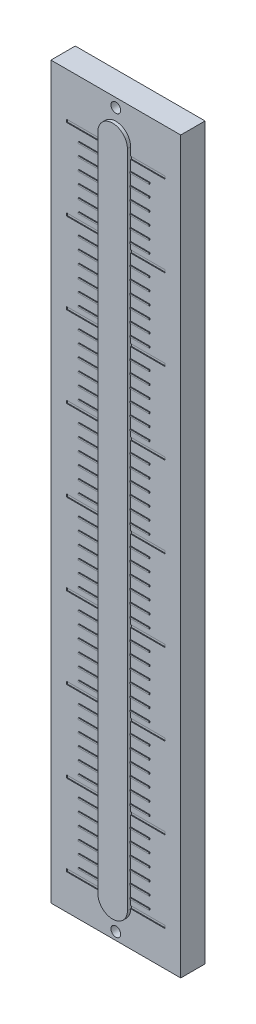
SolidWorks part; units mm, degrees
ref_plane "Front Plane" through (0, 0, 0) normal (0, 0, 1) x (1, 0, 0)
ref_plane "Top Plane" through (0, 0, 0) normal (0, 1, 0) x (1, 0, 0)
ref_plane "Right Plane" through (0, 0, 0) normal (1, 0, 0) x (0, 0, -1)
other "Configuration Table"
sketch "Sketch1" plane through (0, 0, 0) normal (0, 0, 1) x (1, 0, 0)
  line L1 (0, 0) -> (80, 0)
  line L2 (0, 0) -> (0, 450)
  line L3 (0, 450) -> (80, 450)
  line L4 (80, 0) -> (80, 450)
  circle A0 centre (40, 444.6132) radius 3
  circle A1 centre (40, 4.8019) radius 3
  dimension "D3" = 6
  dimension "D4" = 6
  dimension "D1" = 80
  dimension "D2" = 450
extrude "Boss-Extrude1" add sketch "Sketch1" along normal blind 15
sketch "Sketch2" plane through (0, 0, 15) normal (0, 0, 1) x (1, 0, 0)
  line L0 (40.0265, 428.2428) -> (40.0265, 21.5201) construction
  line L1 (49.1252, 428.2428) -> (49.1252, 21.5201)
  line L2 (30.9278, 428.2428) -> (30.9278, 21.5201)
  arc A0 (49.1252, 428.2428) -> (30.9278, 428.2428) centre (40.0265, 428.2428) ccw
  arc A1 (30.9278, 21.5201) -> (49.1252, 21.5201) centre (40.0265, 21.5201) ccw
  point P2 (40.0265, 224.8815)
extrude "Boss-Extrude2" add sketch "Sketch2" along normal blind 2
sketch "Sketch4" plane through (0, 0, 15) normal (0, 0, 1) x (1, 0, 0)
  line L0 (49.1252, 71.5201) -> (49.1252, 73.266)
  line L1 (49.1252, 21.5201) -> (70.4543, 21.5201)
  line L2 (49.1252, 21.5201) -> (49.1252, 23.266)
  line L3 (49.1252, 23.266) -> (70.4543, 23.266)
  line L4 (70.4543, 21.5201) -> (70.4543, 23.266)
  line L5 (49.1252, 71.5201) -> (70.4543, 71.5201)
  line L6 (70.4543, 71.5201) -> (70.4543, 73.266)
  line L7 (49.1252, 73.266) -> (70.4543, 73.266)
  line L8 (49.1252, 121.5201) -> (49.1252, 123.266)
  line L9 (49.1252, 121.5201) -> (70.4543, 121.5201)
  line L10 (70.4543, 121.5201) -> (70.4543, 123.266)
  line L11 (49.1252, 123.266) -> (70.4543, 123.266)
  line L12 (49.1252, 171.5201) -> (49.1252, 173.266)
  line L13 (49.1252, 171.5201) -> (70.4543, 171.5201)
  line L14 (70.4543, 171.5201) -> (70.4543, 173.266)
  line L15 (49.1252, 173.266) -> (70.4543, 173.266)
  line L16 (49.1252, 221.5201) -> (49.1252, 223.266)
  line L17 (49.1252, 221.5201) -> (70.4543, 221.5201)
  line L18 (70.4543, 221.5201) -> (70.4543, 223.266)
  line L19 (49.1252, 223.266) -> (70.4543, 223.266)
  line L20 (49.1252, 271.5201) -> (49.1252, 273.266)
  line L21 (49.1252, 271.5201) -> (70.4543, 271.5201)
  line L22 (70.4543, 271.5201) -> (70.4543, 273.266)
  line L23 (49.1252, 273.266) -> (70.4543, 273.266)
  line L24 (49.1252, 321.5201) -> (49.1252, 323.266)
  line L25 (49.1252, 321.5201) -> (70.4543, 321.5201)
  line L26 (70.4543, 321.5201) -> (70.4543, 323.266)
  line L27 (49.1252, 323.266) -> (70.4543, 323.266)
  line L28 (49.1252, 371.5201) -> (49.1252, 373.266)
  line L29 (49.1252, 371.5201) -> (70.4543, 371.5201)
  line L30 (70.4543, 371.5201) -> (70.4543, 373.266)
  line L31 (49.1252, 373.266) -> (70.4543, 373.266)
  line L32 (49.1252, 421.5201) -> (49.1252, 423.266)
  line L33 (49.1252, 421.5201) -> (70.4543, 421.5201)
  line L34 (70.4543, 421.5201) -> (70.4543, 423.266)
  line L35 (49.1252, 423.266) -> (70.4543, 423.266)
  line L36 (30.9278, 71.5201) -> (30.9278, 73.266)
  line L37 (30.9278, 21.5201) -> (9.6218, 21.5201)
  line L38 (30.9278, 21.5201) -> (30.9278, 23.266)
  line L39 (30.9278, 23.266) -> (9.6218, 23.266)
  line L40 (9.6218, 21.5201) -> (9.6218, 23.266)
  line L41 (30.9278, 71.5201) -> (9.6218, 71.5201)
  line L42 (9.6218, 71.5201) -> (9.6218, 73.266)
  line L43 (30.9278, 73.266) -> (9.6218, 73.266)
  line L44 (30.9278, 121.5201) -> (30.9278, 123.266)
  line L45 (30.9278, 121.5201) -> (9.6218, 121.5201)
  line L46 (9.6218, 121.5201) -> (9.6218, 123.266)
  line L47 (30.9278, 123.266) -> (9.6218, 123.266)
  line L48 (30.9278, 171.5201) -> (30.9278, 173.266)
  line L49 (30.9278, 171.5201) -> (9.6218, 171.5201)
  line L50 (9.6218, 171.5201) -> (9.6218, 173.266)
  line L51 (30.9278, 173.266) -> (9.6218, 173.266)
  line L52 (30.9278, 221.5201) -> (30.9278, 223.266)
  line L53 (30.9278, 221.5201) -> (9.6218, 221.5201)
  line L54 (9.6218, 221.5201) -> (9.6218, 223.266)
  line L55 (30.9278, 223.266) -> (9.6218, 223.266)
  line L56 (30.9278, 271.5201) -> (30.9278, 273.266)
  line L57 (30.9278, 271.5201) -> (9.6218, 271.5201)
  line L58 (9.6218, 271.5201) -> (9.6218, 273.266)
  line L59 (30.9278, 273.266) -> (9.6218, 273.266)
  line L60 (30.9278, 321.5201) -> (30.9278, 323.266)
  line L61 (30.9278, 321.5201) -> (9.6218, 321.5201)
  line L62 (9.6218, 321.5201) -> (9.6218, 323.266)
  line L63 (30.9278, 323.266) -> (9.6218, 323.266)
  line L64 (30.9278, 371.5201) -> (30.9278, 373.266)
  line L65 (30.9278, 371.5201) -> (9.6218, 371.5201)
  line L66 (9.6218, 371.5201) -> (9.6218, 373.266)
  line L67 (30.9278, 373.266) -> (9.6218, 373.266)
  line L68 (30.9278, 421.5201) -> (30.9278, 423.266)
  line L69 (30.9278, 421.5201) -> (9.6218, 421.5201)
  line L70 (9.6218, 421.5201) -> (9.6218, 423.266)
  line L71 (30.9278, 423.266) -> (9.6218, 423.266)
  dimension "D1" = 9
  dimension "D2" = 9
extrude "Cut-Extrude1" cut sketch "Sketch4" against normal blind 0.5
sketch "Sketch5" plane through (0, 0, 15) normal (0, 0, 1) x (1, 0, 0)
  line L0 (17.3259, 35.2703) -> (17.3259, 34.3689)
  line L1 (17.3259, 27.7703) -> (60.981, 27.7703)
  line L2 (17.3259, 27.7703) -> (17.3259, 26.8689)
  line L3 (17.3259, 26.8689) -> (60.981, 26.8689)
  line L4 (60.981, 27.7703) -> (60.981, 26.8689)
  line L5 (17.3259, 35.2703) -> (60.981, 35.2703)
  line L6 (60.981, 35.2703) -> (60.981, 34.3689)
  line L7 (17.3259, 34.3689) -> (60.981, 34.3689)
  line L8 (17.3259, 42.7703) -> (17.3259, 41.8689)
  line L9 (17.3259, 42.7703) -> (60.981, 42.7703)
  line L10 (60.981, 42.7703) -> (60.981, 41.8689)
  line L11 (17.3259, 41.8689) -> (60.981, 41.8689)
  line L12 (17.3259, 50.2703) -> (17.3259, 49.3689)
  line L13 (17.3259, 50.2703) -> (60.981, 50.2703)
  line L14 (60.981, 50.2703) -> (60.981, 49.3689)
  line L15 (17.3259, 49.3689) -> (60.981, 49.3689)
  line L16 (17.3259, 57.7703) -> (17.3259, 56.8689)
  line L17 (17.3259, 57.7703) -> (60.981, 57.7703)
  line L18 (60.981, 57.7703) -> (60.981, 56.8689)
  line L19 (17.3259, 56.8689) -> (60.981, 56.8689)
  line L20 (17.3259, 65.2703) -> (17.3259, 64.3689)
  line L21 (17.3259, 65.2703) -> (60.981, 65.2703)
  line L22 (60.981, 65.2703) -> (60.981, 64.3689)
  line L23 (17.3259, 64.3689) -> (60.981, 64.3689)
  dimension "D1" = 6
extrude "Boss-Extrude3" add sketch "Sketch5" along normal blind 0.5
pattern_linear "LPattern1" count 8 spacing 50 along (0, 1, 0) of "Boss-Extrude3"
